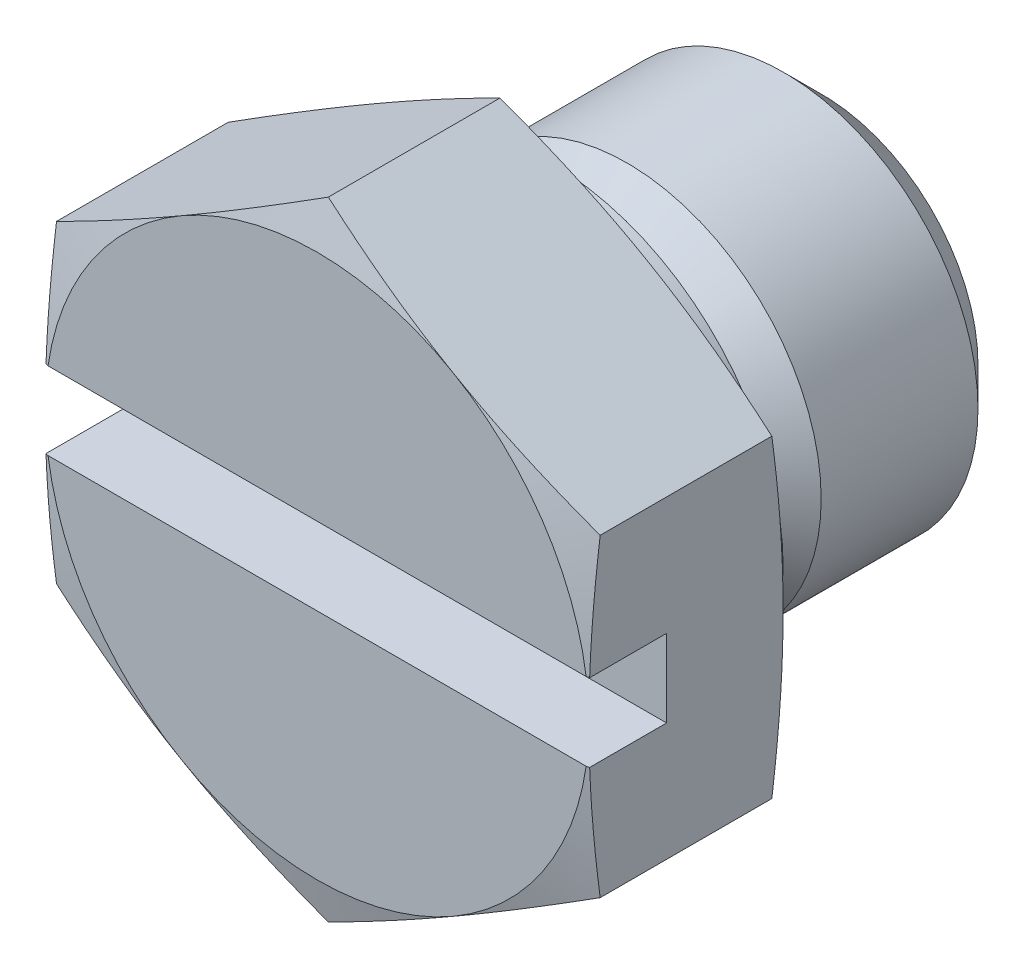
from build123d import *

# Parameters (mm, degrees)
SKETCH2_R          = 5
CUT_EXTRUDE1_DEPTH = 3
SKETCH3_W          = 10
SKETCH3_H          = 1
CUT_EXTRUDE2_DEPTH = 1


with BuildPart() as part:
    # Sketch1 → Revolve1 (revolve)
    with BuildSketch(Plane(origin=(0, 0, 0), x_dir=(0, 0, -1), z_dir=(1, 0, 0)), mode=Mode.PRIVATE) as revolve1_sk:
        Polygon((-3, 0), (-3, 3.5), (-2.598076211, 5), (-0.901923789, 5), (-0.5, 3.5), (-0.5, 3), (0, 3), (0, 2.2), (0.5, 2.2), (0.5, 2.0095), (0.9905, 2.5), (3.0095, 2.5), (3.5, 2.0095), (3.5, 0), align=None)
    revolve(revolve1_sk.sketch.rotate(Axis((0, 0, -3.5), (0, 0, 1)), 270), axis=Axis((0, 0, -3.5), (0, 0, 1)))

    # Sketch2 → Cut-Extrude1 (cut)
    with BuildSketch(Plane.XY):
        Circle(SKETCH2_R)
        Polygon((-3.5, 2.020725942), (-3.5, -2.020725942), (0, -4.041451884), (3.5, -2.020725942), (3.5, 2.020725942), (0, 4.041451884), align=None, mode=Mode.SUBTRACT)
    extrude(amount=CUT_EXTRUDE1_DEPTH, mode=Mode.SUBTRACT)

    # Sketch3 → Cut-Extrude2 (cut)
    with BuildSketch(Plane.XY.offset(3)):
        Rectangle(SKETCH3_W, SKETCH3_H)
    extrude(amount=-CUT_EXTRUDE2_DEPTH, mode=Mode.SUBTRACT)


solid = part.part
